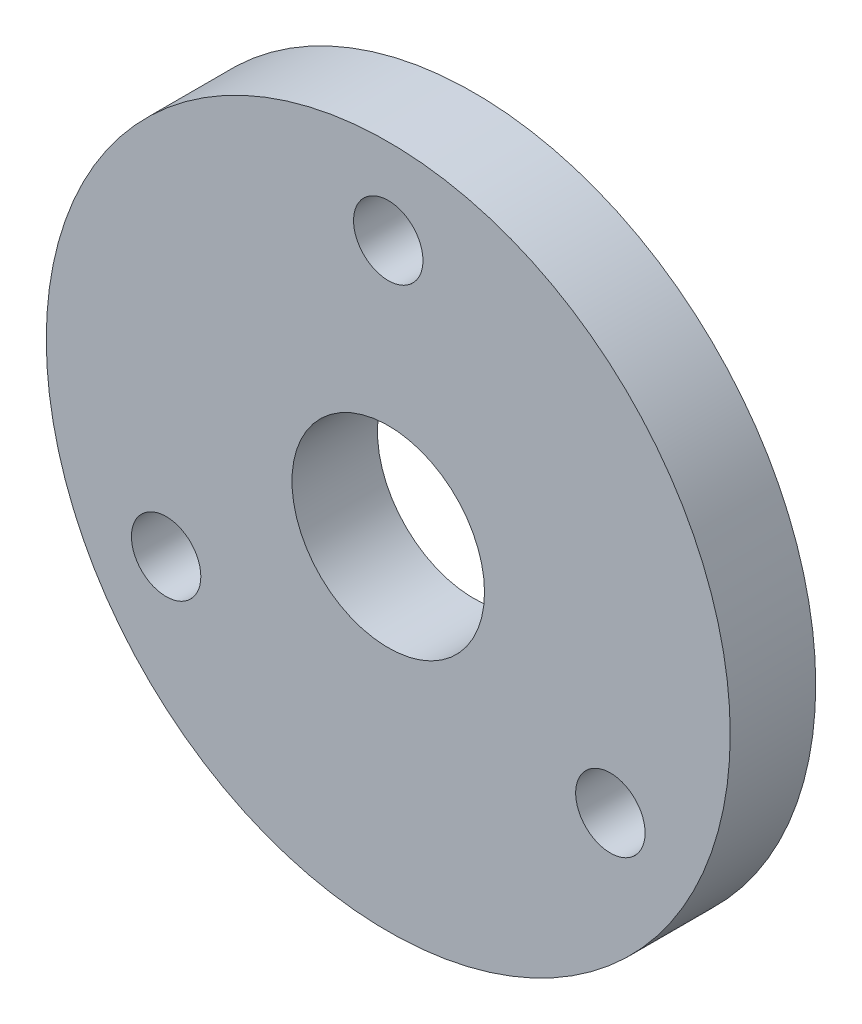
SolidWorks part; units mm, degrees
ref_plane "Front Plane" through (0, 0, 0) normal (0, 0, 1) x (1, 0, 0)
ref_plane "Top Plane" through (0, 0, 0) normal (0, 1, 0) x (1, 0, 0)
ref_plane "Right Plane" through (0, 0, 0) normal (1, 0, 0) x (0, 0, -1)
sketch "Sketch1" plane through (0, 0, 0) normal (0, 0, 1) x (1, 0, 0)
  circle A0 centre (0, 0) radius 25.4
  circle A1 centre (0, 0) radius 7.1501
  dimension "D1" = 50.8
  dimension "D2" = 14.3002
extrude "Boss-Extrude1" add sketch "Sketch1" against normal blind 6.35
sketch "Sketch2" plane through (0, 0, 0) normal (0, 0, 1) x (1, 0, 0)
  line L0 (0, 0) -> (0, 19.05) construction
  line L1 (0, 0) -> (16.4978, -9.525) construction
  circle A0 centre (0, 0) radius 19.05 construction
  circle A1 centre (0, 19.05) radius 2.5781
  circle A2 centre (16.4978, -9.525) radius 2.5781
  circle A3 centre (0, 0) radius 19.05 construction
  circle A4 centre (-16.4978, -9.525) radius 2.5781
  circle A5 centre (0, 0) radius 19.05 construction
  dimension "D1" = 38.1
  dimension "D2" = 5.1562
  dimension "D4" = 120
  dimension "D3" = 3
extrude "Cut-Extrude1" cut sketch "Sketch2" against normal blind 6.35
